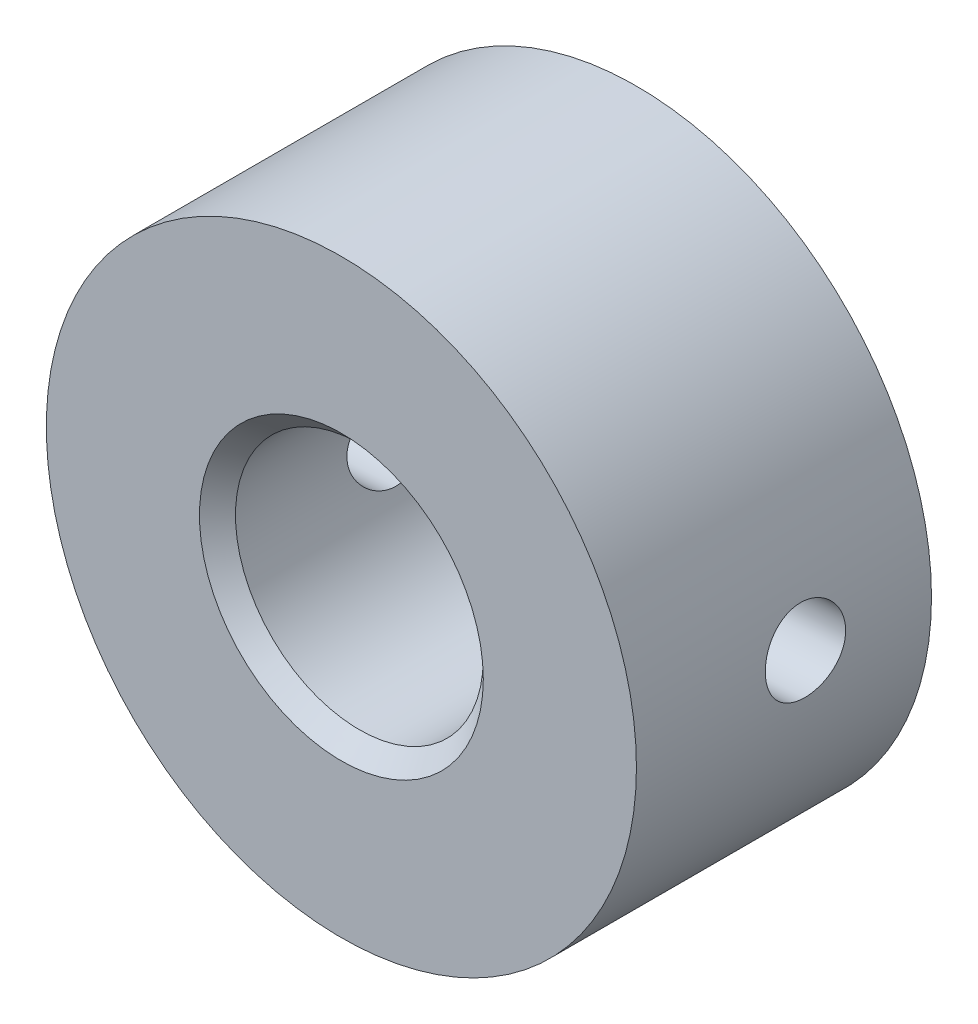
SolidWorks part; units mm, degrees
ref_plane "Front Plane" through (0, 0, 0) normal (0, 0, 1) x (1, 0, 0)
ref_plane "Top Plane" through (0, 0, 0) normal (0, 1, 0) x (1, 0, 0)
ref_plane "Right Plane" through (0, 0, 0) normal (1, 0, 0) x (0, 0, -1)
other "Configuration Table"
sketch "Sketch1" plane through (0, 0, 0) normal (0, 0, 1) x (1, 0, 0)
  circle A0 centre (0, 0) radius 25
  dimension "D1" = 50
extrude "Boss-Extrude1" add sketch "Sketch1" along normal blind 25
hole_wizard "M24 Tapped Hole1" positions "3DSketch1" profile "Sketch2" tap size "M24" standard "GB"
sketch3d "3DSketch1"
  line L0 (0, 0, 25) -> (0, 0, 0) construction
  point P0 (0, 0, 25)
sketch "Sketch2" plane through (0, 0, 25) normal (1, 0, 0) x (0, -1, 0)
  line L0 (0, 0) -> (0, 63.309)
  line L1 (0, 63.309) -> (10.5, 57)
  line L2 (10.5, 57) -> (10.5, 1.525)
  line L3 (10.5, 1.525) -> (12.025, 0)
  line L5 (12.025, 0) -> (0, 0)
  line L6 (-10.5, 1.525) -> (-12.025, 0) construction
  line L10 (0, 63.309) -> (-10.5, 57) construction
  line L11 (0, -6.35) -> (0, 107.95) construction
  dimension "螺纹孔钻头直径" = 21
  dimension "螺纹孔钻头深度" = 57
  dimension "近端锥形沉头孔直径" = 24.05
  dimension "近端锥形沉头孔角度" = 90
  dimension "导头角度" = 118
cosmetic thread "Hole Thread1" parameters "D1"=48, "D2"=24
hole_wizard "M8 Tapped Hole1" positions "3DSketch2" profile "Sketch3" tap size "M8" standard "GB"
sketch3d "3DSketch2"
  point P0 (-24.9655, -1.3135, 10.6434)
sketch "Sketch3" plane through (-24.9655, -1.3135, 10.6434) normal (0, 0, 1) x (0.0525, -0.9986, 0)
  line L0 (0, 0) -> (0, 65.7929)
  line L1 (0, 65.7929) -> (3.4, 63.75)
  line L2 (3.4, 63.75) -> (3.4, 0.625)
  line L3 (3.4, 0.625) -> (4.025, 0)
  line L5 (4.025, 0) -> (0, 0)
  line L6 (-3.4, 0.625) -> (-4.025, 0) construction
  line L10 (0, 65.7929) -> (-3.4, 63.75) construction
  line L11 (0, -6.35) -> (0, 107.95) construction
  dimension "螺纹孔钻头直径" = 6.8
  dimension "螺纹孔钻头深度" = 63.75
  dimension "近端锥形沉头孔直径" = 8.05
  dimension "近端锥形沉头孔角度" = 90
  dimension "导头角度" = 118
cosmetic thread "Hole Thread2" parameters "D1"=60, "D2"=8
